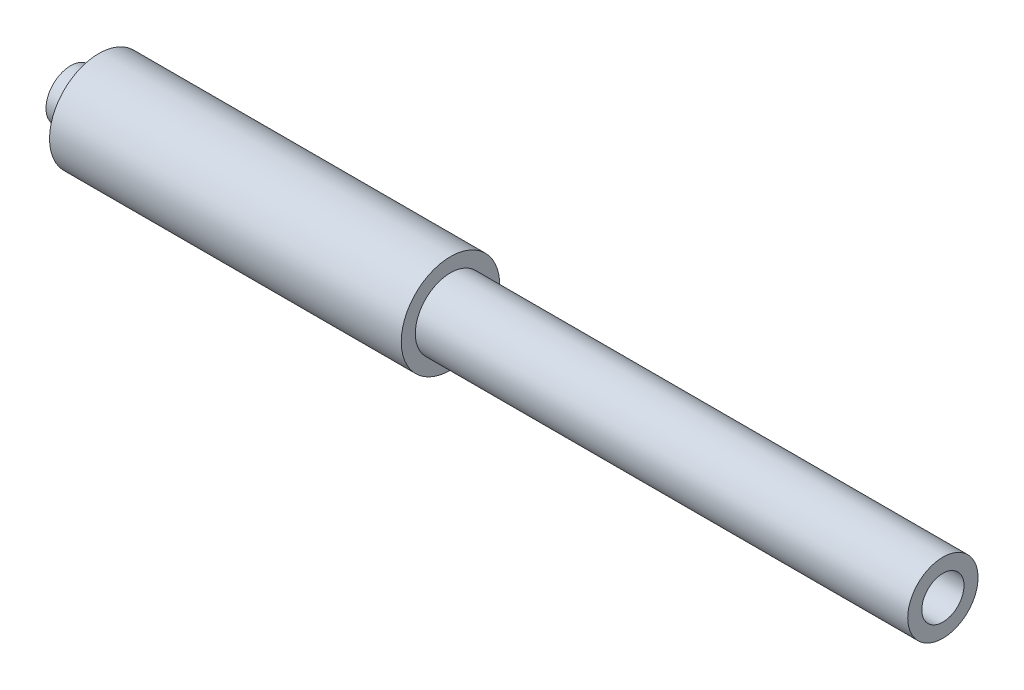
SolidWorks part; units mm, degrees
material "普通碳钢"
ref_plane "Front Plane" through (0, 0, 0) normal (0, 0, 1) x (1, 0, 0)
ref_plane "Top Plane" through (0, 0, 0) normal (0, 1, 0) x (1, 0, 0)
ref_plane "Right Plane" through (0, 0, 0) normal (1, 0, 0) x (0, 0, -1)
sketch "Sketch1" plane through (0, 0, 0) normal (0, 0, 1) x (1, 0, 0)
  line L0 (-12.5607, 193.2845) -> (709.3843, 193.2845) construction
  line L1 (631.1739, 208.2845) -> (631.1739, 218.2845)
  line L2 (631.1739, 218.2845) -> (281.1739, 218.2845)
  line L3 (281.1739, 218.2845) -> (281.1739, 228.2845)
  line L4 (281.1739, 228.2845) -> (31.1739, 228.2845)
  line L5 (31.1739, 228.2845) -> (31.1739, 210.7845)
  line L6 (41.1739, 218.2845) -> (271.1739, 218.2845)
  line L7 (271.1739, 218.2845) -> (271.1739, 208.2845)
  line L8 (271.1739, 208.2845) -> (631.1739, 208.2845)
  line L9 (11.1739, 200.7845) -> (41.1739, 200.7845)
  line L10 (41.1739, 200.7845) -> (41.1739, 218.2845)
  line L11 (11.1739, 200.7845) -> (11.1739, 210.7845)
  line L13 (11.1739, 210.7845) -> (31.1739, 210.7845)
  dimension "D2" = 10
  dimension "D3" = 25
  dimension "D4" = 25
  dimension "D5" = 10
  dimension "D6" = 350
  dimension "D7" = 620
  dimension "D8" = 250
  dimension "D9" = 10
  dimension "D10" = 10
revolve "Revolve1" add sketch "Sketch1" angle 360 about L0
